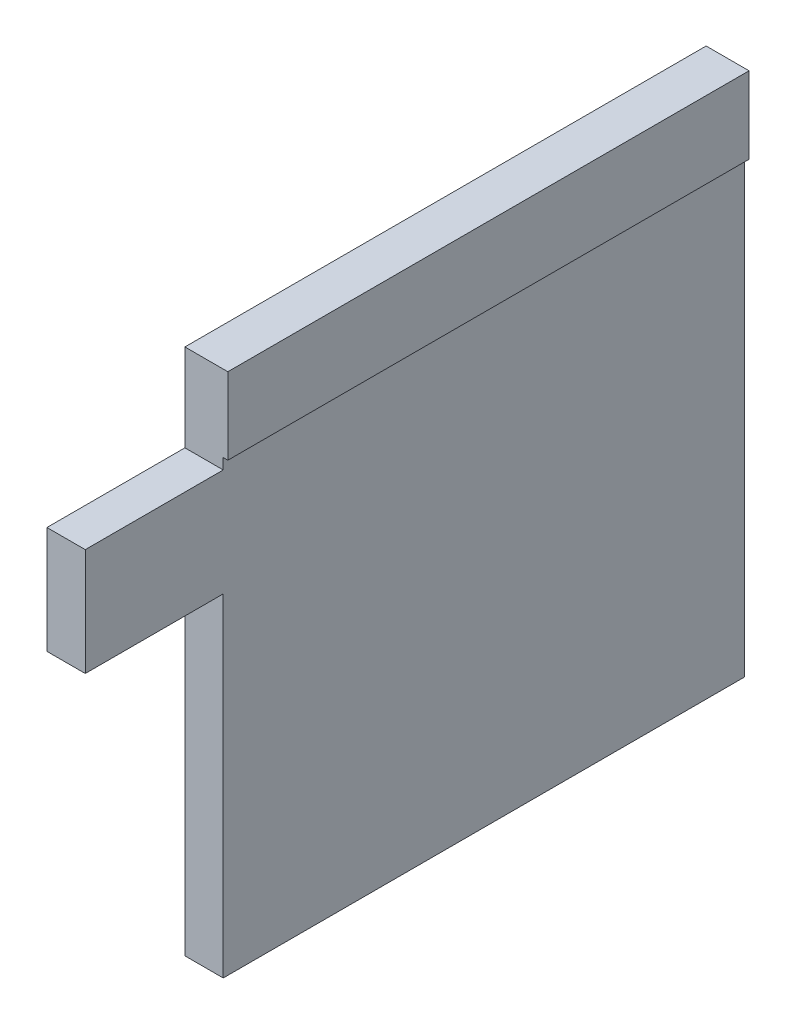
from build123d import *

# Parameters (mm, degrees)
EXTRUDE_1_DEPTH = 85
SKETCH_4_W      = 12.5
SKETCH_4_H      = 35
EXTRUDE_2_DEPTH = 45


with BuildPart() as part:
    # 草图1 → 凸台-拉伸1 (new, symmetric)
    with BuildSketch(Plane.XY):
        Polygon((0, 0), (0, 172), (14, 172), (14, 147), (12.5, 147), (12.5, 0), align=None)
    extrude(amount=EXTRUDE_1_DEPTH, both=True)

    # 草图4 → 凸台-拉伸2 (add)
    with BuildSketch(Plane(origin=(0, 0, 85), x_dir=(-1, 0, 0), z_dir=(0, 0, -1))):
        with Locations((-6.25, 126)):
            Rectangle(SKETCH_4_W, SKETCH_4_H)
    extrude(amount=-EXTRUDE_2_DEPTH)


solid = part.part
